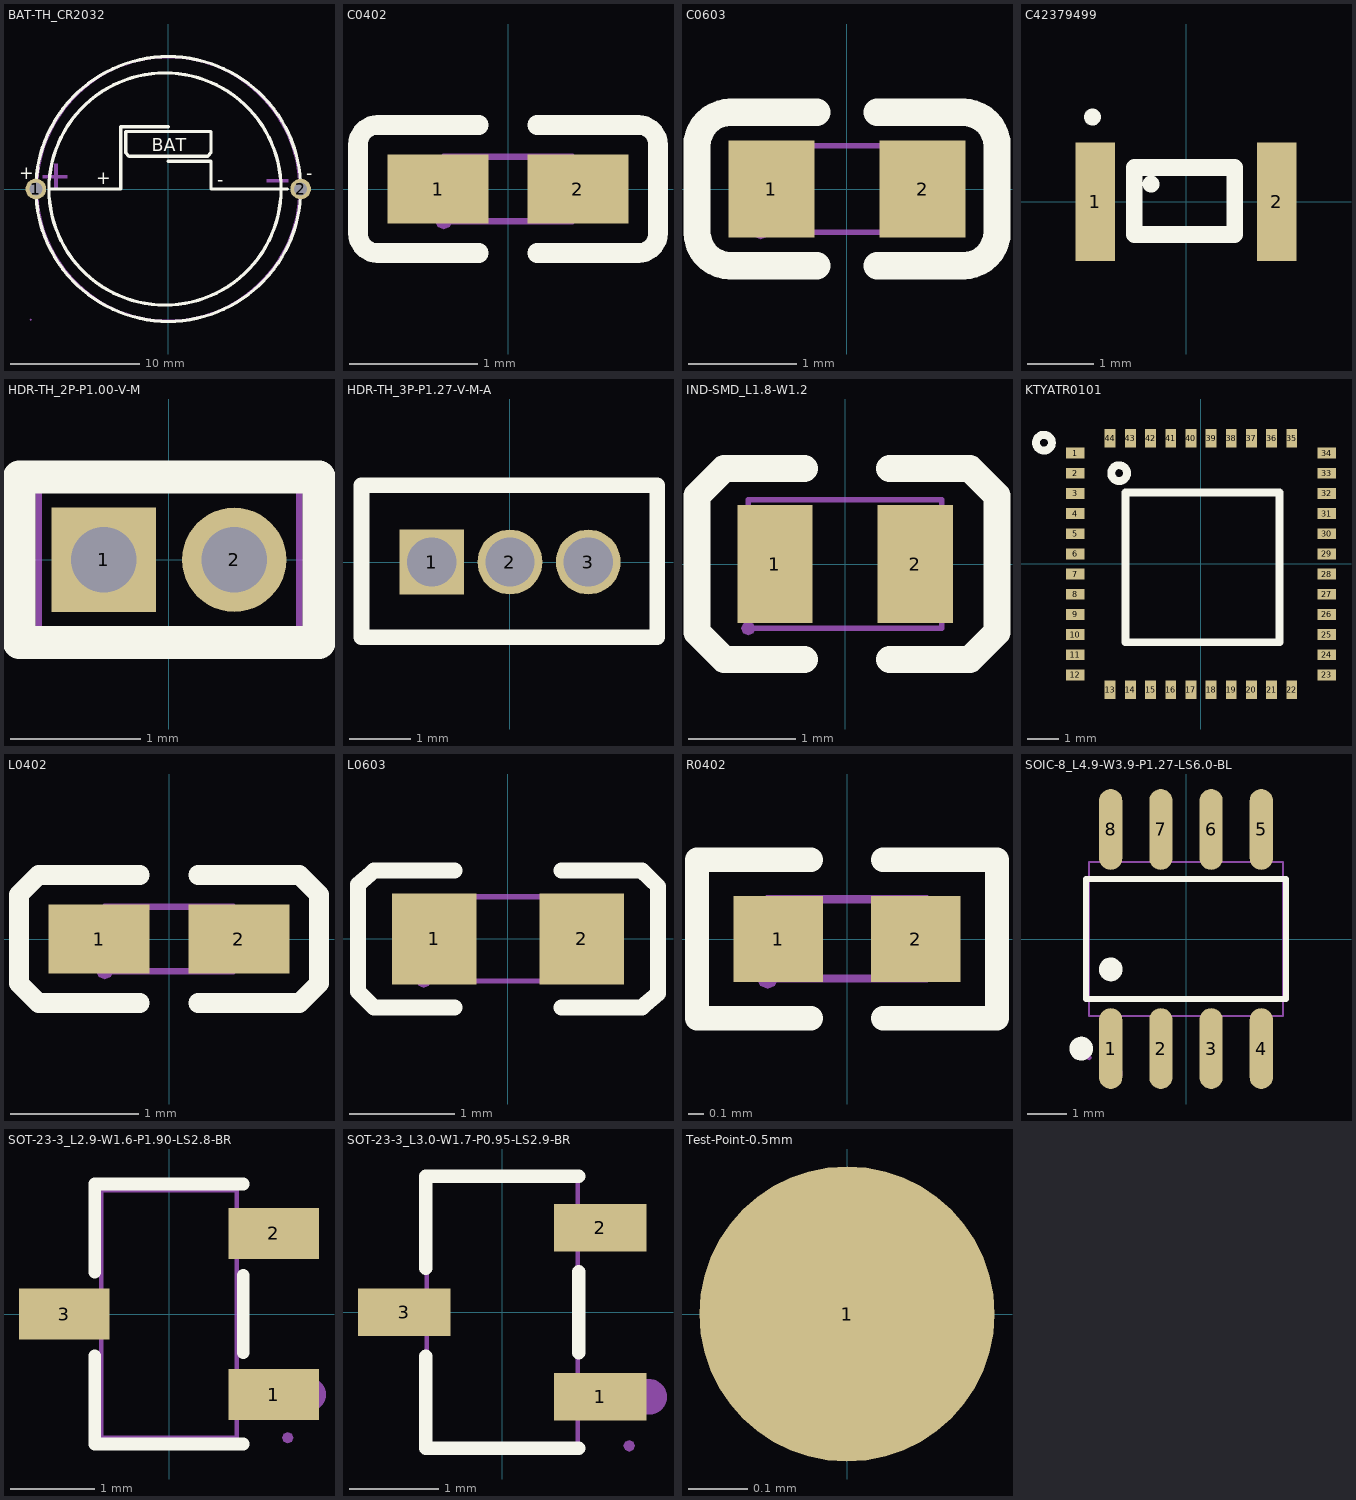
[diagram p0: the footprints below, top view; thin cyan lines are the x and y axes]
# Altium footprint library MISC82703-9.PcbLib: 15 footprints
Each footprint in its own frame and in the unit in brackets; x right, y up, seen from the top. Pads: shape width x height; smd on the part's side, far side on the other; paste and mask are expansions set on the pad; w line width, h text height; cw(c..) or ccw(c..) is an arc to the next point about the centre after c.

## BAT-TH_CR2032 [mm]
pads (2):
  round 1.6 hole 1: 1(-10.25,0) 2(10.25,0)
Top Overlay:
  circle w0.254: c0,0 r10.25
  circle w0.254: c-0.254,0 r8.988
  lines w0.254: -9.219,0 -3.683,0 -3.683,0.889 -3.683,4.826 0,4.826 ; 0,2.159 3.302,2.159 3.302,0.889 3.302,0 9.219,0 ; 3.175,2.667 3.302,2.794 ; 3.302,2.794 3.302,4.445 -3.302,4.445 -3.302,2.794 -3.048,2.54 3.048,2.54 3.302,2.794
  text "-" at 3.81,0.254 h1
  text "+" at -5.588,0.381 h1
  text "BAT" at -1.27,2.921 h1
  text "-" at 10.668,0.762 h1
  text "+" at -11.557,0.762 h1
Mechanical 6:
  region: 7.62,0.762 7.62,0.508 9.271,0.508 9.271,0.762
  region: -9.716,1.079 -9.716,0.826 -8.826,0.826 -8.826,0.064 -8.572,0.064 -8.572,0.826 -7.81,0.826 -7.81,1.079 -8.572,1.079 -8.572,1.968 -8.826,1.968 -8.826,1.079
Mechanical 15:
  region: 9.843,0 9.873,0.15 9.962,0.282 10.094,0.371 10.25,0.402 10.406,0.371 10.538,0.282 10.627,0.15 10.656,0 10.627,-0.15 10.538,-0.282 10.406,-0.371 10.25,-0.402 10.094,-0.371 9.962,-0.282 9.873,-0.15
  region: -10.656,0 -10.627,0.15 -10.538,0.282 -10.406,0.371 -10.25,0.402 -10.094,0.371 -9.962,0.282 -9.873,0.15 -9.843,0 -9.873,-0.15 -9.962,-0.282 -10.094,-0.371 -10.25,-0.402 -10.406,-0.371 -10.538,-0.282 -10.627,-0.15
  region: -10.715,-10.127 -10.696,-10.081 -10.65,-10.062 -10.604,-10.081 -10.585,-10.127 -10.604,-10.173 -10.65,-10.192 -10.696,-10.173 -10.715,-10.127
  lines w0.051: -10.127,0 ccw(c0,0) 10.127,0 ccw(c0,0) -10.127,0

## C0402 [mm]
pads (2):
  rect 0.79x0.54 smd paste-100 mask+0.051: 1(-0.545,0) 2(0.545,0)
Top Overlay:
  lines w0.152: -0.226,-0.499 -1.016,-0.499 cw(c-1.016,-0.346) -1.169,-0.346 -1.169,0.346 cw(c-1.016,0.346) -1.016,0.499 -0.226,0.499 ; 0.226,-0.499 1.016,-0.499 ccw(c1.016,-0.346) 1.169,-0.346 1.169,0.346 ccw(c1.016,0.346) 1.016,0.499 0.226,0.499
Top Paste:
  region: 0.78,0.225 0.78,-0.225 0.73,-0.275 0.25,-0.275 0.18,-0.225 0.18,0.225 0.25,0.275 0.73,0.275
  region: -0.18,0.225 -0.18,-0.225 -0.25,-0.275 -0.73,-0.275 -0.78,-0.225 -0.78,0.225 -0.73,0.275 -0.25,0.275
Mechanical 15:
  region: 0.5,-0.25 0.5,0.25 0.25,0.25 0.25,-0.25
  region: -0.5,-0.25 -0.5,0.25 -0.25,0.25 -0.25,-0.25
  region: -0.565,-0.25 -0.546,-0.296 -0.5,-0.315 -0.454,-0.296 -0.435,-0.25 -0.454,-0.204 -0.5,-0.185 -0.546,-0.204
  lines w0.051: -0.5,-0.25 0.5,-0.25 0.5,0.25 -0.5,0.25 -0.5,-0.25

## C0603 [mm]
pads (2):
  rect 0.8x0.9 smd: 1(-0.7,0) 2(0.7,0)
Top Overlay:
  lines w0.254: -1.08,-0.71 -0.28,-0.71 ; -1.08,0.71 -0.28,0.71 ; -1.08,-0.71 cw(c-1.08,-0.4) -1.39,-0.4 -1.39,0.4 cw(c-1.08,0.4) -1.08,0.71 ; 0.28,-0.71 1.08,-0.71 ccw(c1.08,-0.4) 1.39,-0.4 1.39,0.4 ccw(c1.08,0.4) 1.08,0.71 0.28,0.71
Mechanical 15:
  region: 0.8,-0.4 0.8,0.4 0.5,0.4 0.5,-0.4
  region: -0.8,-0.4 -0.8,0.4 -0.5,0.4 -0.5,-0.4
  region: -0.736,-0.4 -0.754,-0.355 -0.8,-0.336 -0.846,-0.355 -0.865,-0.4 -0.846,-0.445 -0.8,-0.464 -0.754,-0.445
  lines w0.051: -0.8,-0.4 0.8,-0.4 0.8,0.4 -0.8,0.4 -0.8,-0.4

## C42379499 [mm]
pads (2):
  rect 0.6x1.8 smd: 1(-1.374,0) 2(1.374,0)
Top Overlay:
  circle w0.254: c-1.42,1.281 r0.003
  circle w0.254: c-0.531,0.265 r0.003
  lines w0.254: -0.785,-0.497 -0.785,0.519 0.739,0.519 0.739,-0.497 -0.785,-0.497

## HDR-TH_2P-P1.00-V-M [mm]
pads (2):
  rect 0.8x0.8 hole 0.5 paste+0 mask+0.05: 1(-0.5,0)
  round 0.8 hole 0.5 paste+0 mask+0.05: 2(0.5,0)
Top Overlay:
  lines w0.254: -1.15,-0.635 1.15,-0.635 1.15,0.635 -1.15,0.635 -1.15,-0.635
Mechanical 15:
  region: 0.35,-0.15 0.35,0.15 0.65,0.15 0.65,-0.15
  region: -0.65,-0.15 -0.65,0.15 -0.35,0.15 -0.35,-0.15
  region: -0.935,-0.635 -0.954,-0.589 -1,-0.57 -1.046,-0.589 -1.065,-0.635 -1.046,-0.681 -1,-0.7 -0.954,-0.681 -0.935,-0.635
  lines w0.051: -1,-0.635 1,-0.635 1,0.635 -1,0.635 -1,-0.635

## HDR-TH_3P-P1.27-V-M-A [mm]
pads (3):
  rect 1.05x1.05 hole 0.8: 1(-1.27,0)
  round 1.05 hole 0.8: 2(0,0) 3(1.27,0)
Top Overlay:
  lines w0.254: -2.408,-1.222 -2.408,1.243 2.389,1.243 2.389,-1.222 -2.408,-1.222
Mechanical 15:
  region: 1.02,0.25 1.52,0.25 1.52,-0.25 1.02,-0.25
  region: -0.25,0.25 0.25,0.25 0.25,-0.25 -0.25,-0.25
  region: -1.52,0.25 -1.02,0.25 -1.02,-0.25 -1.52,-0.25
  region: -2.4,-1.314 -2.355,-1.296 -2.336,-1.25 -2.355,-1.204 -2.4,-1.185 -2.4,-1.186 -2.445,-1.204 -2.464,-1.25 -2.445,-1.296
  lines w0.051: -2.4,-1.25 2.4,-1.25 2.4,1.25 -2.4,1.25 -2.4,-1.25

## IND-SMD_L1.8-W1.2 [mm]
pads (2):
  rect 0.7x1.1 smd: 1(-0.653,0) 2(0.653,0)
Top Overlay:
  lines w0.254: -0.381,-0.889 -1.125,-0.889 -1.379,-0.635 -1.379,0.635 -1.125,0.889 -0.381,0.889 ; 0.417,-0.889 1.161,-0.889 1.415,-0.635 1.415,0.635 1.161,0.889 0.417,0.889
Mechanical 15:
  region: 0.487,0.45 0.817,0.45 0.817,-0.45 0.487,-0.45
  region: -0.818,0.45 -0.488,0.45 -0.488,-0.45 -0.818,-0.45
  region: -0.9,-0.665 -0.854,-0.646 -0.835,-0.6 -0.854,-0.554 -0.9,-0.535 -0.946,-0.554 -0.965,-0.6 -0.946,-0.646
  lines w0.051: -0.9,-0.6 0.9,-0.6 0.9,0.6 -0.9,0.6 -0.9,-0.6

## KTYATR0101 [mm]
pads (44):
  rect 0.6x0.35 smd: 1(-4.05,3.575) 2(-4.05,2.925) 3(-4.05,2.275) 4(-4.05,1.625) 5(-4.05,0.975) 6(-4.05,0.325) 7(-4.05,-0.325) 8(-4.05,-0.975) 9(-4.05,-1.625) 10(-4.05,-2.275) 11(-4.05,-2.925) 12(-4.05,-3.575) 23(4.05,-3.575) 24(4.05,-2.925) 25(4.05,-2.275) 26(4.05,-1.625) 27(4.05,-0.975) 28(4.05,-0.325) 29(4.05,0.325) 30(4.05,0.975) 31(4.05,1.625) 32(4.05,2.275) 33(4.05,2.925) 34(4.05,3.575)
  rect 0.35x0.6 smd: 13(-2.925,-4.05) 14(-2.275,-4.05) 15(-1.625,-4.05) 16(-0.975,-4.05) 17(-0.325,-4.05) 18(0.325,-4.05) 19(0.975,-4.05) 20(1.625,-4.05) 21(2.275,-4.05) 22(2.925,-4.05) 35(2.925,4.05) 36(2.275,4.05) 37(1.625,4.05) 38(0.975,4.05) 39(0.325,4.05) 40(-0.325,4.05) 41(-0.975,4.05) 42(-1.625,4.05) 43(-2.275,4.05) 44(-2.925,4.05)
Top Overlay:
  circle w0.254: c-5.059,3.908 r0.256
  circle w0.254: c-2.637,2.927 r0.256
  lines w0.254: -2.427,-2.521 -2.427,2.305 2.526,2.305 2.526,-2.521 -2.427,-2.521

## L0402 [mm]
pads (2):
  rect 0.79x0.54 smd paste-100 mask+0.051: 1(-0.545,0) 2(0.545,0)
Top Overlay:
  lines w0.152: -0.226,-0.499 -1.016,-0.499 -1.169,-0.346 -1.169,0.346 -1.016,0.499 -0.226,0.499 ; 0.226,-0.499 1.016,-0.499 1.169,-0.346 1.169,0.346 1.016,0.499 0.226,0.499
Top Paste:
  region: -0.135,-0.086 -0.135,0.086 -0.404,0.27 -0.9,0.27 -0.94,0.23 -0.94,-0.23 -0.9,-0.27 -0.404,-0.27
  region: 0.135,-0.086 0.135,0.086 0.404,0.27 0.9,0.27 0.94,0.23 0.94,-0.23 0.9,-0.27 0.404,-0.27
Mechanical 15:
  region: 0.5,-0.25 0.5,0.25 0.25,0.25 0.25,-0.25
  region: -0.5,-0.25 -0.5,0.25 -0.25,0.25 -0.25,-0.25
  region: -0.5,-0.315 -0.454,-0.296 -0.435,-0.25 -0.454,-0.204 -0.5,-0.185 -0.546,-0.204 -0.565,-0.25 -0.546,-0.296
  lines w0.051: -0.5,-0.25 0.5,-0.25 0.5,0.25 -0.5,0.25 -0.5,-0.25

## L0603 [mm]
pads (2):
  rect 0.8x0.864 smd paste-100 mask+0.051: 1(-0.7,0) 2(0.7,0)
Top Overlay:
  lines w0.152: -1.272,-0.65 -0.51,-0.65 ; -1.272,0.65 -0.51,0.65 ; -1.27,-0.651 -1.424,-0.499 -1.424,0.517 -1.27,0.65 ; 0.51,-0.65 1.272,-0.65 ; 0.51,0.65 1.272,0.65 ; 1.27,-0.65 1.424,-0.517 1.424,0.499 1.27,0.65
Top Paste:
  region: -0.252,0.143 -0.252,-0.134 -0.526,-0.427 -1.029,-0.427 -1.093,-0.363 -1.093,0.373 -1.029,0.437 -0.526,0.437
  region: 0.264,0.154 0.264,-0.122 0.538,-0.416 1.042,-0.416 1.106,-0.352 1.106,0.384 1.042,0.448 0.538,0.448
Mechanical 15:
  region: -0.865,-0.4 -0.846,-0.446 -0.8,-0.465 -0.754,-0.446 -0.735,-0.4 -0.754,-0.354 -0.8,-0.335 -0.846,-0.354 -0.865,-0.4
  region: 0.8,-0.4 0.5,-0.4 0.5,0.4 0.8,0.4
  region: -0.5,-0.4 -0.8,-0.4 -0.8,0.4 -0.5,0.4
  lines w0.051: -0.8,-0.4 0.8,-0.4 0.8,0.4 -0.8,0.4 -0.8,-0.4

## R0402 [mm]
pads (2):
  rect 0.566x0.54 smd paste-100 mask+0.051: 1(-0.433,0) 2(0.433,0)
Top Overlay:
  lines w0.152: -0.226,-0.499 -0.944,-0.499 -0.944,0.499 -0.226,0.499 ; 0.226,-0.499 0.944,-0.499 0.944,0.499 0.226,0.499
Top Paste:
  region: -0.135,-0.23 -0.135,0.23 -0.175,0.27 -0.676,0.27 -0.716,0.23 -0.716,-0.23 -0.676,-0.27 -0.175,-0.27
  region: 0.135,-0.23 0.135,0.23 0.175,0.27 0.676,0.27 0.716,0.23 0.716,-0.23 0.676,-0.27 0.175,-0.27
Mechanical 15:
  region: -0.249,0.25 -0.249,-0.25 -0.499,-0.25 -0.499,0.25
  region: 0.251,-0.25 0.251,0.25 0.501,0.25 0.501,-0.25
  region: -0.435,-0.25 -0.454,-0.205 -0.5,-0.186 -0.546,-0.205 -0.564,-0.25 -0.546,-0.295 -0.5,-0.314 -0.454,-0.295
  lines w0.051: -0.5,-0.25 0.5,-0.25 0.5,0.25 -0.5,0.25 -0.5,-0.25

## SOIC-8_L4.9-W3.9-P1.27-LS6.0-BL [mm]
pads (8):
  oval 0.588x2.045 smd: 1(-1.905,-2.772) 2(-0.635,-2.772) 3(0.635,-2.772) 4(1.905,-2.772) 5(1.905,2.772) 6(0.635,2.772) 7(-0.635,2.772) 8(-1.905,2.772)
Top Overlay:
  circle w0.3: c-2.652,-2.772 r0.15
  circle w0.3: c-1.905,-0.769 r0.15
  lines w0.152: -2.526,-1.521 2.526,-1.521 2.526,1.521 -2.526,1.521 -2.526,-1.521
Mechanical 6:
  circle w0.3: c-1.905,-3.4 r0.15
Mechanical 15:
  region: 1.695,2.175 1.695,1.94 2.115,1.94 2.115,2.175
  region: 1.695,3 1.695,2.165 2.115,2.165 2.115,3
  region: 0.425,2.175 0.425,1.94 0.845,1.94 0.845,2.175
  region: 0.425,3 0.425,2.165 0.845,2.165 0.845,3
  region: -0.845,2.175 -0.845,1.94 -0.425,1.94 -0.425,2.175
  region: -0.845,3 -0.845,2.165 -0.425,2.165 -0.425,3
  region: -2.115,2.175 -2.115,1.94 -1.695,1.94 -1.695,2.175
  region: -2.115,3 -2.115,2.165 -1.695,2.165 -1.695,3
  region: 1.695,-2.175 1.695,-1.94 2.115,-1.94 2.115,-2.175
  region: 1.695,-3 1.695,-2.165 2.115,-2.165 2.115,-3
  region: 0.425,-2.175 0.425,-1.94 0.845,-1.94 0.845,-2.175
  region: 0.425,-3 0.425,-2.165 0.845,-2.165 0.845,-3
  region: -0.845,-2.175 -0.845,-1.94 -0.425,-1.94 -0.425,-2.175
  region: -0.845,-3 -0.845,-2.165 -0.425,-2.165 -0.425,-3
  region: -2.115,-2.175 -2.115,-1.94 -1.695,-1.94 -1.695,-2.175
  region: -2.115,-3 -2.115,-2.165 -1.695,-2.165 -1.695,-3
  region: -2.45,-2.936 -2.495,-2.954 -2.514,-3 -2.495,-3.046 -2.45,-3.064 -2.405,-3.046 -2.386,-3 -2.405,-2.954
  lines w0.051: -2.45,-1.95 2.45,-1.95 2.45,1.95 -2.45,1.95 -2.45,-1.95

## SOT-23-3_L2.9-W1.6-P1.90-LS2.8-BR [mm]
pads (3):
  rect 1.07x0.6 smd: 1(1.235,-0.95) 2(1.235,0.95) 3(-1.235,0)
Top Overlay:
  lines w0.152: -0.876,-0.495 -0.876,-1.536 0.876,-1.536 ; -0.876,0.495 -0.876,1.536 0.876,1.536 ; 0.876,-0.455 0.876,0.455
Mechanical 6:
  circle w0.2: c1.651,-0.95 r0.1
Mechanical 15:
  region: -0.96,-0.2 -0.96,0.2 -0.79,0.2 -0.79,-0.2
  region: -0.95,-0.2 -0.95,0.2 -1.4,0.2 -1.4,-0.2
  region: 0.79,0.75 0.79,1.15 0.96,1.15 0.96,0.75
  region: 0.95,0.75 0.95,1.15 1.4,1.15 1.4,0.75
  region: 0.79,-1.15 0.79,-0.75 0.96,-0.75 0.96,-1.15
  region: 0.95,-1.15 0.95,-0.75 1.4,-0.75 1.4,-1.15
  region: 1.335,-1.46 1.354,-1.414 1.4,-1.395 1.446,-1.414 1.465,-1.46 1.446,-1.506 1.4,-1.525 1.354,-1.506 1.335,-1.46
  lines w0.051: -0.8,-1.46 0.8,-1.46 0.8,1.46 -0.8,1.46 -0.8,-1.46

## SOT-23-3_L3.0-W1.7-P0.95-LS2.9-BR [mm]
pads (3):
  rect 1.037x0.532 smd: 1(1.101,-0.95) 2(1.101,0.95) 3(-1.101,0)
Top Overlay:
  lines w0.152: -0.859,-0.495 -0.859,-1.526 0.859,-1.526 ; -0.859,0.495 -0.859,1.526 0.859,1.526 ; 0.859,-0.455 0.859,0.455
Mechanical 6:
  circle w0.2: c1.65,-0.95 r0.1
Mechanical 15:
  region: 1,-1.137 1,-0.762 1.425,-0.762 1.425,-1.137
  region: 0.815,-1.137 0.815,-0.762 1.01,-0.762 1.01,-1.137
  region: 1,0.762 1,1.137 1.425,1.137 1.425,0.762
  region: 0.815,0.762 0.815,1.137 1.01,1.137 1.01,0.762
  region: -1.425,-0.188 -1.425,0.188 -1,0.188 -1,-0.188
  region: -1.01,-0.188 -1.01,0.188 -0.815,0.188 -0.815,-0.188
  region: 1.425,-1.435 1.47,-1.454 1.489,-1.5 1.47,-1.546 1.425,-1.564 1.38,-1.546 1.361,-1.5 1.38,-1.454
  lines w0.051: -0.85,-1.5 -0.85,1.5 0.85,1.5 0.85,-1.5 -0.85,-1.5

## Test-Point-0.5mm [mm]
pads (1):
  round 0.5 smd: 1(0,0)